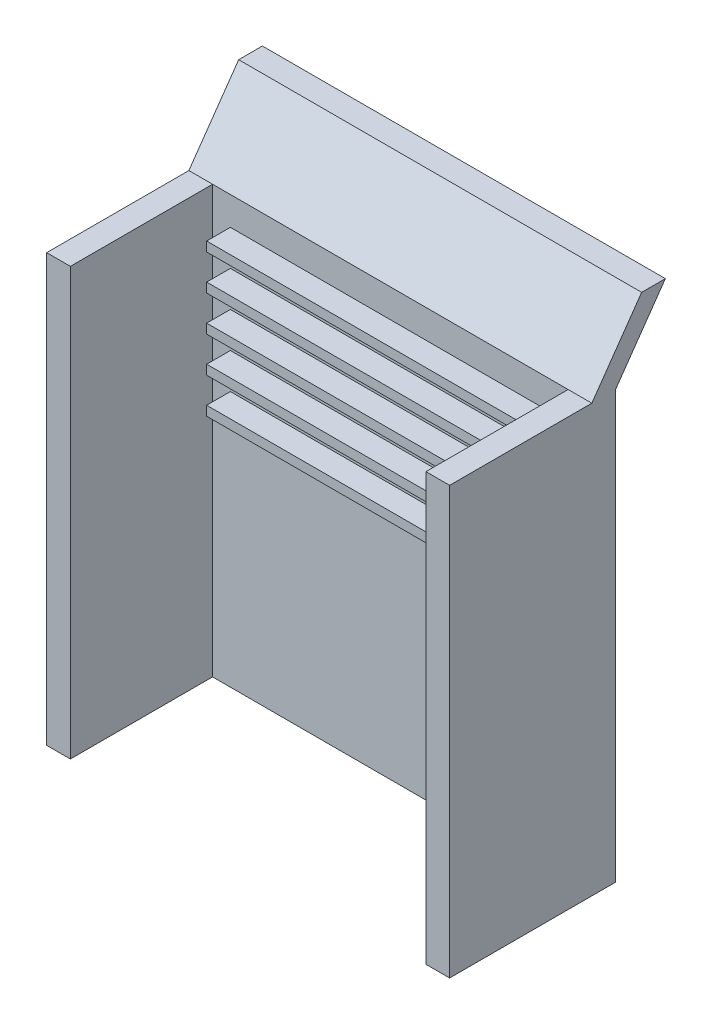
SolidWorks part; units mm, degrees
ref_plane "前视基准面" through (0, 0, 0) normal (0, 0, 1) x (1, 0, 0)
ref_plane "上视基准面" through (0, 0, 0) normal (0, 1, 0) x (1, 0, 0)
ref_plane "右视基准面" through (0, 0, 0) normal (1, 0, 0) x (0, 0, -1)
sketch "草图1" plane through (0, 0, 0) normal (0, 0, 1) x (1, 0, 0)
  line L1 (-85, -90) -> (85, -90)
  line L2 (-85, -90) -> (-85, 90)
  line L3 (-85, 90) -> (85, 90)
  line L4 (85, -90) -> (85, 90)
  line L5 (-85, -90) -> (85, 90) construction
  line L6 (-85, 90) -> (85, -90) construction
  point P0 (0, 0)
  dimension "D1" = 170
  dimension "D2" = 180
extrude "凸台-拉伸1" add sketch "草图1" along normal blind 10
sketch "草图2" plane through (0, 0, 10) normal (0, 0, 1) x (1, 0, 0)
  line L0 (-85, -90) -> (85, -90) construction
  line L1 (-85, 90) -> (-75, 90)
  line L2 (-85, 90) -> (-85, -90)
  line L3 (-85, -90) -> (-75, -90)
  line L4 (-75, 90) -> (-75, -90)
  line L6 (85, 90) -> (75, 90)
  line L7 (85, 90) -> (85, -90)
  line L8 (85, -90) -> (75, -90)
  line L9 (75, 90) -> (75, -90)
  dimension "D1" = 10
extrude "凸台-拉伸2" add sketch "草图2" along normal blind 60
sketch "草图3" plane through (85, 0, 0) normal (1, 0, 0) x (0, 0, -1)
  line L0 (0, 90) -> (21.0062, 120)
  line L1 (21.0062, 120) -> (11.0062, 120)
  line L2 (11.0062, 120) -> (-10, 90)
  line L3 (-70, 90) -> (0, 90) construction
  line L4 (-10, 90) -> (0, 90)
  line L5 (0, -90) -> (0, 90) construction
  dimension "D1" = 10
  dimension "D2" = 145
  dimension "D3" = 30
extrude "凸台-拉伸3" add sketch "草图3" against normal up to surface (170 mm away) up to face at (-85, 0, 35)
sketch "草图4" plane through (0, 0, 10) normal (0, 0, 1) x (1, 0, 0)
  line L0 (0, 0) -> (0, 90) construction
  line L1 (75, 90) -> (-75, 90) construction
  line L3 (-67.5, 74) -> (67.5, 74)
  line L4 (-67.5, 74) -> (-67.5, 78)
  line L5 (-67.5, 78) -> (67.5, 78)
  line L6 (67.5, 74) -> (67.5, 78)
  line L7 (-67.5, 74) -> (67.5, 78) construction
  line L8 (-67.5, 78) -> (67.5, 74) construction
  point P5 (0, 76)
  dimension "D1" = 135
  dimension "D2" = 4
  dimension "D3" = 12
extrude "凸台-拉伸4" add sketch "草图4" along normal blind 10
pattern_linear "阵列(线性)1" count 5 spacing 15 along (0, -1, 0) of "凸台-拉伸4"
